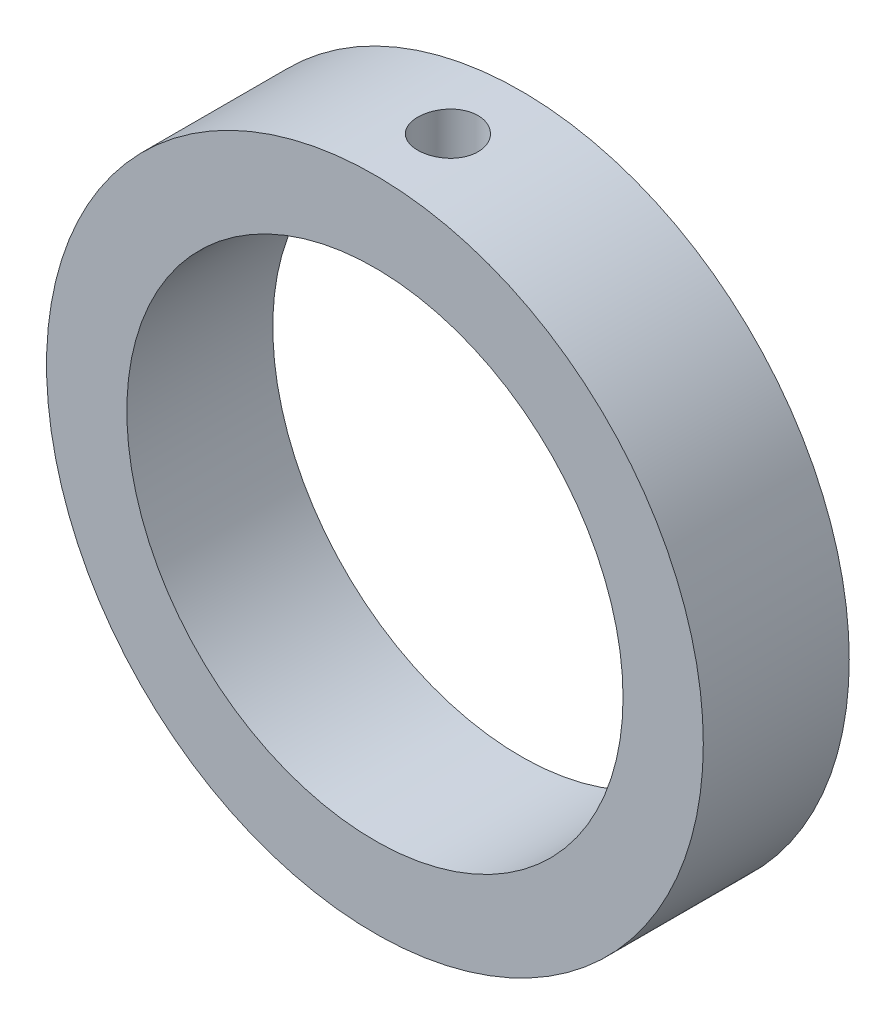
SolidWorks part; units mm, degrees
ref_plane "前视基准面" through (0, 0, 0) normal (0, 0, 1) x (1, 0, 0)
ref_plane "上视基准面" through (0, 0, 0) normal (0, 1, 0) x (1, 0, 0)
ref_plane "右视基准面" through (0, 0, 0) normal (1, 0, 0) x (0, 0, -1)
sketch "草图1" plane through (0, 0, 0) normal (0, 0, 1) x (1, 0, 0)
  circle A0 centre (0, 0) radius 13.6
  circle A1 centre (0, 0) radius 18
  dimension "D1" = 27.2
  dimension "D2" = 36
extrude "凸台-拉伸1" add sketch "草图1" along normal mid plane 8
hole_wizard "M4 螺纹孔2" positions "草图7" profile "草图8" tap size "M4" standard "GB"
sketch "草图7" plane through (0, 0, 0) normal (0, 1, 0) x (1, 0, 0)
  point P0 (0, 0)
sketch "草图8" plane through (0, 0, 0) normal (1, 0, 0) x (0, 0, -1)
  line L0 (0, 0) -> (0, 18)
  line L1 (0, 18) -> (1.65, 18)
  line L2 (1.65, 18) -> (1.65, 0)
  line L5 (1.65, 0) -> (0, 0)
  line L11 (0, -6.35) -> (0, 107.95) construction
  dimension "通孔螺纹孔钻头直径" = 3.3
  dimension "通孔螺纹孔钻头深度" = 18
cosmetic thread "孔螺蚊线3" parameters "D2"=4
